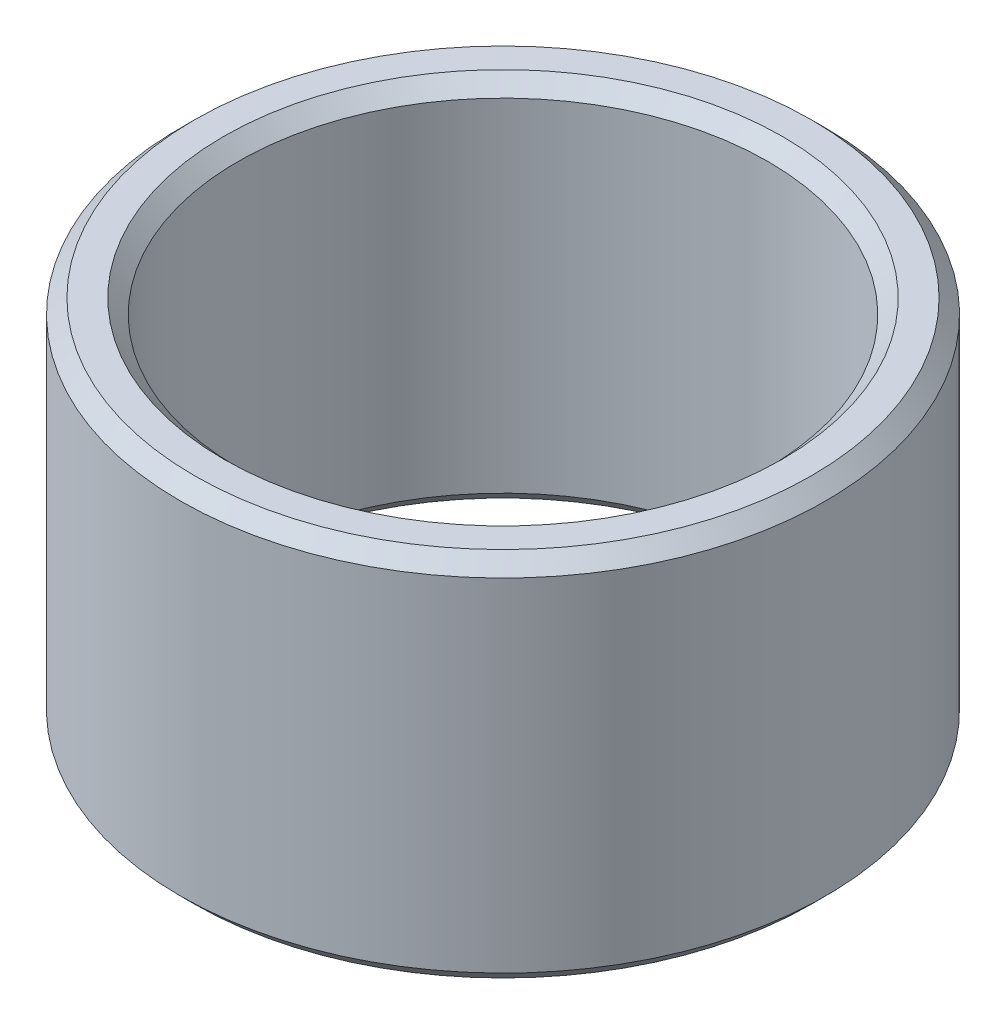
from build123d import *

# Parameters (mm, degrees)
SKETCH1_R           = 33.5
SKETCH1_R_2         = 27.5
BOSS_EXTRUDE1_DEPTH = 38.5
CHAMFER1_SIZE       = 1.5


with BuildPart() as part:
    # Sketch1 → Boss-Extrude1 (new body)
    with BuildSketch(Plane(origin=(0, 0, 0), x_dir=(1, 0, 0), z_dir=(0, 1, 0))):
        with Locations(Location((0, 0, 0), (0, 0, 270))):
            Circle(SKETCH1_R)
        with Locations(Location((0, 0, 0), (0, 0, 270))):
            Circle(SKETCH1_R_2, mode=Mode.SUBTRACT)
    extrude(amount=BOSS_EXTRUDE1_DEPTH)

    # Chamfer1
    chamfer1_edges = [part.edges().sort_by_distance(p)[0] for p in [
        (0, 0, -33.5),
        (0, 38.5, -33.5),
        (0, 0, -27.5),
        (0, 38.5, -27.5),
    ]]
    chamfer(chamfer1_edges, length=CHAMFER1_SIZE)


solid = part.part
